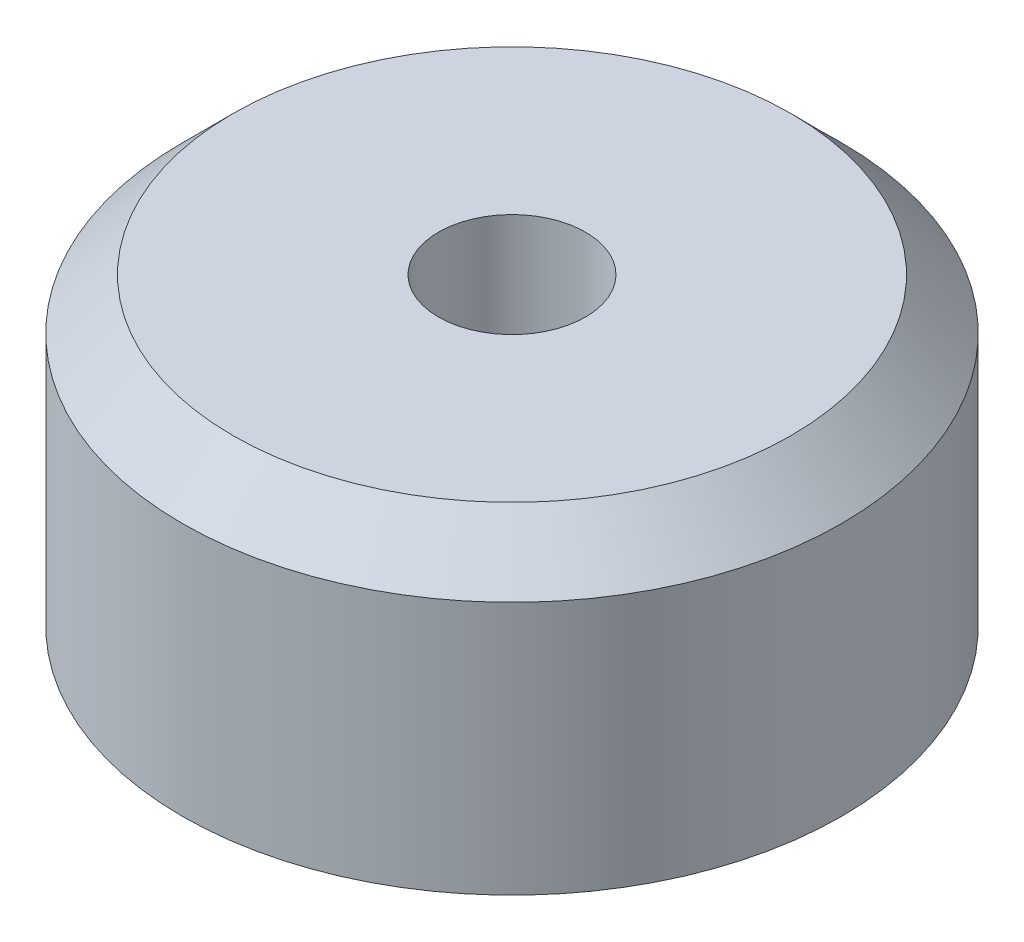
from build123d import *

# Parameters (mm, degrees)
SKETCH1_R                  = 32.5
BOSS_EXTRUDE1_DEPTH        = 30
CHAMFER1_SIZE              = 5
M16X1_5_TAPPED_HOLE1_D     = 14.5
M16X1_5_TAPPED_HOLE1_DEPTH = 36.5
M16X1_5_TAPPED_HOLE1_TIP   = 4.356239488


with BuildPart() as part:
    # Sketch1 → Boss-Extrude1 (new body)
    with BuildSketch(Plane(origin=(0, 0, 0), x_dir=(1, 0, 0), z_dir=(0, 1, 0))):
        with Locations(Location((0, 0, 0), (0, 0, 270))):
            Circle(SKETCH1_R)
    extrude(amount=BOSS_EXTRUDE1_DEPTH)

    # Chamfer1
    chamfer1_edges = [part.edges().sort_by_distance(p)[0] for p in [
        (0, 30, -32.5),
    ]]
    chamfer(chamfer1_edges, length=CHAMFER1_SIZE)

    # M16x1.5 Tapped Hole1
    with Locations(Plane(origin=(0, 30, 0), x_dir=(1, 0, 0), z_dir=(0, 1, 0))):
        with Locations((0, 0)):
            Hole(M16X1_5_TAPPED_HOLE1_D / 2, depth=M16X1_5_TAPPED_HOLE1_DEPTH)
            with Locations((0, 0, -(M16X1_5_TAPPED_HOLE1_DEPTH + M16X1_5_TAPPED_HOLE1_TIP / 2))):  # 118° drill point
                Cone(0, M16X1_5_TAPPED_HOLE1_D / 2, M16X1_5_TAPPED_HOLE1_TIP, mode=Mode.SUBTRACT)


solid = part.part
